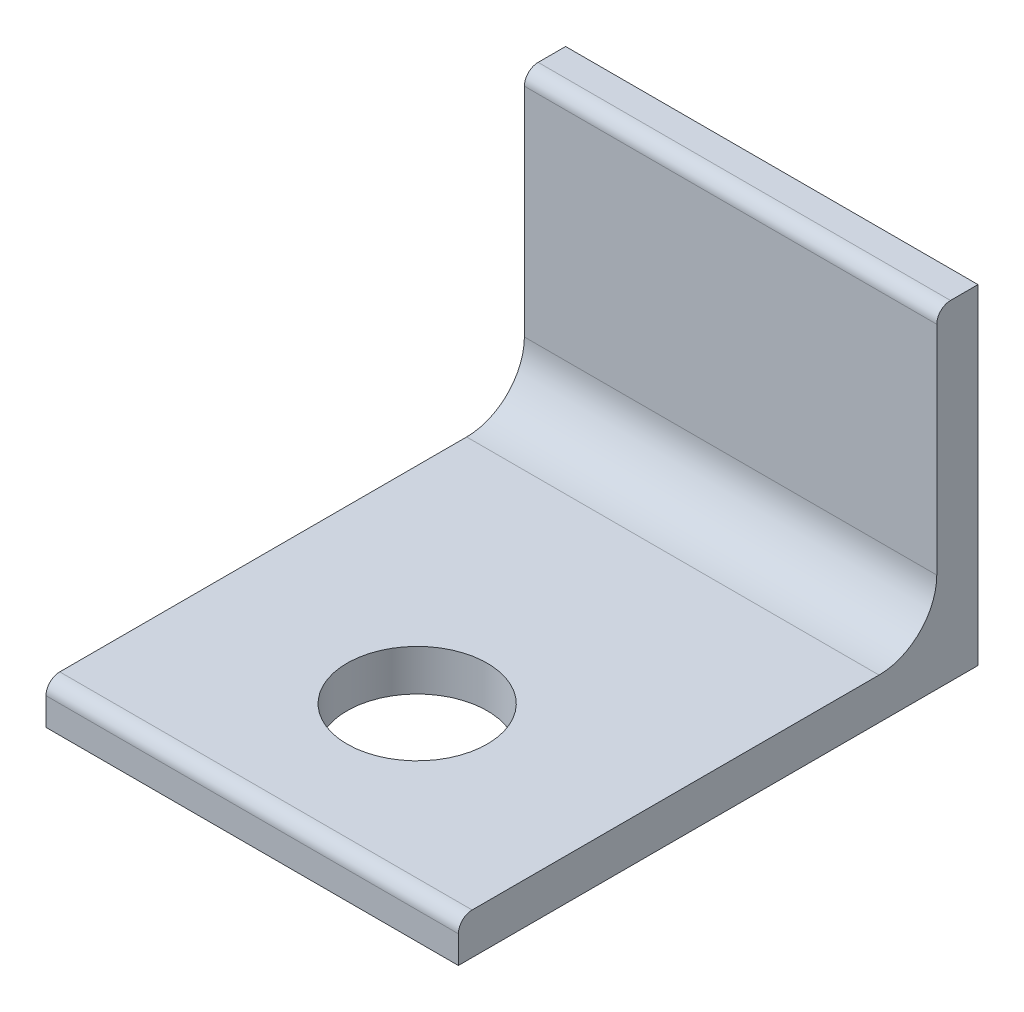
SolidWorks part; units mm, degrees
material "Q235"
ref_plane "Front" through (0, 0, 0) normal (0, 0, 1) x (1, 0, 0)
ref_plane "Top" through (0, 0, 0) normal (0, 1, 0) x (1, 0, 0)
ref_plane "Right" through (0, 0, 0) normal (1, 0, 0) x (0, 0, -1)
sketch "草图1" plane through (0, 0, 0) normal (0, 0, 1) x (1, 0, 0)
  line L0 (0, 0) -> (50, 0)
  dimension "D1" = 50
other "Unequal Angle 6.3-4-5(1)"
ref_plane "Plane1" through (0, 0, 0) normal (1, 0, 0) x (0, 0, 1)
sketch "Sketch1" plane through (0, 0, 0) normal (1, 0, 0) x (0, 0, 1)
  line L0 (63, 0) -> (0, 0)
  line L1 (0, 0) -> (0, -40)
  line L2 (61.3333, -5) -> (12, -5)
  line L3 (5, -12) -> (5, -38.3333)
  line L4 (63, 0) -> (63, -3.3333)
  line L5 (0, -40) -> (3.3333, -40)
  arc A0 (63, -3.3333) -> (61.3333, -5) centre (61.3333, -3.3333) cw
  arc A1 (3.3333, -40) -> (5, -38.3333) centre (3.3333, -38.3333) ccw
  arc A2 (12, -5) -> (5, -12) centre (12, -12) ccw
  point P2 (0, -20)
  point P13 (31.5, 0)
  point P14 (0, 0)
  dimension "r1" = 1.6667
  dimension "r" = 7
  dimension "a" = 63
  dimension "d" = 5
  dimension "b" = 40
sketch "Sketch3" plane through (0, 5, 0) normal (0, 1, 0) x (1, 0, 0)
  line L0 (25, -63) -> (25, -43) construction
  line L1 (50, -63) -> (0, -63) construction
  circle A0 centre (25, -43) radius 8.5
  dimension "D1" = 17
  dimension "D2" = 20
extrude "Cut-Extrude1" cut sketch "Sketch3" against normal blind 10
